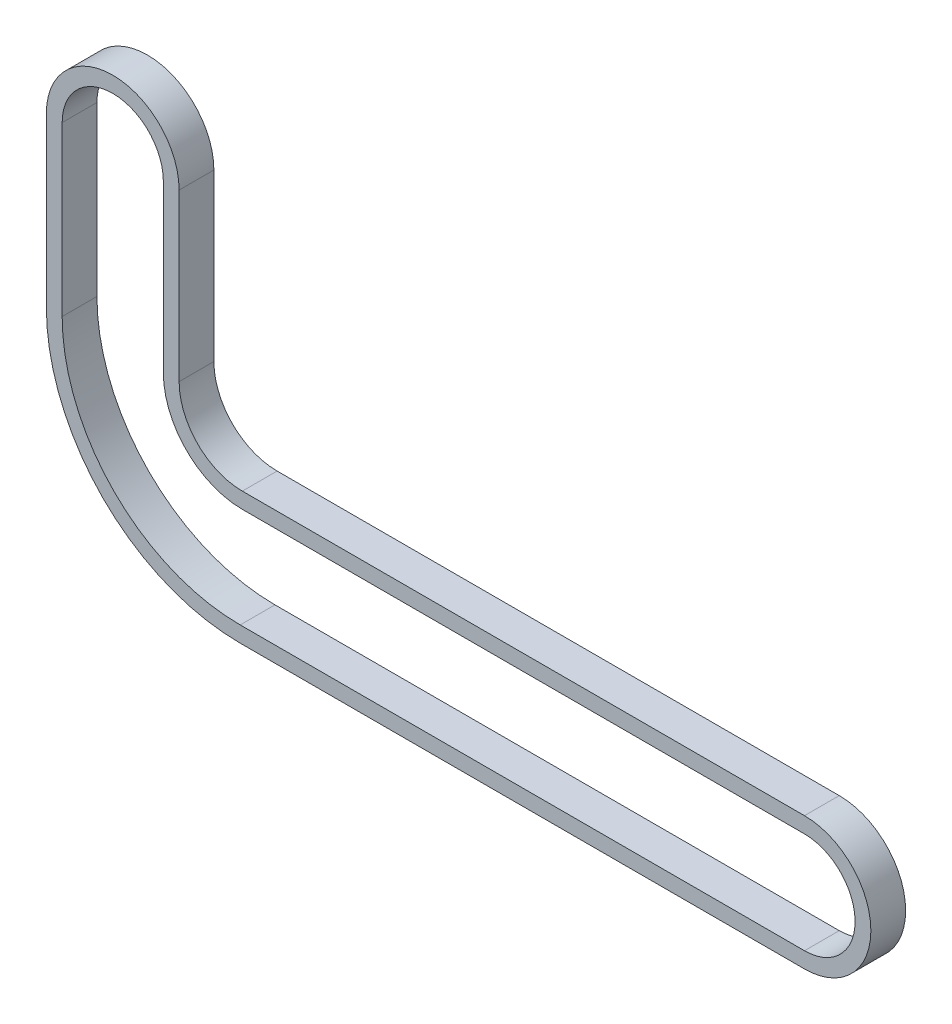
SolidWorks part; units mm, degrees
ref_plane "Front Plane" through (0, 0, 0) normal (0, 0, 1) x (1, 0, 0)
ref_plane "Top Plane" through (0, 0, 0) normal (0, 1, 0) x (1, 0, 0)
ref_plane "Right Plane" through (0, 0, 0) normal (1, 0, 0) x (0, 0, -1)
sketch "Sketch1" plane through (0, 0, 0) normal (0, 0, 1) x (1, 0, 0)
  line L0 (-55.3634, 75.858) -> (-55.3634, 22.7074)
  line L1 (0.9629, -33.6189) -> (179.4809, -33.6189)
  line L3 (179.4809, -1.6189) -> (1.6366, -1.6189)
  line L4 (-23.3634, 23.3811) -> (-23.3634, 75.858)
  line L5 (-18.3634, 23.3811) -> (-18.3634, 75.858)
  line L6 (-60.3634, 75.858) -> (-60.3634, 22.7074)
  line L7 (0.9629, -38.6189) -> (179.4809, -38.6189)
  line L8 (179.4809, 3.3811) -> (1.6366, 3.3811)
  arc A0 (179.4809, -1.6189) -> (179.4809, -33.6189) centre (179.4809, -17.6189) cw
  arc A1 (-55.3634, 22.7074) -> (0.9629, -33.6189) centre (0.9629, 22.7074) ccw
  arc A2 (-55.3634, 75.858) -> (-23.3634, 75.858) centre (-39.3634, 75.858) cw
  arc A3 (1.6366, -1.6189) -> (-23.3634, 23.3811) centre (1.6366, 23.3811) cw
  arc A4 (-60.3634, 75.858) -> (-18.3634, 75.858) centre (-39.3634, 75.858) cw
  arc A5 (-60.3634, 22.7074) -> (0.9629, -38.6189) centre (0.9629, 22.7074) ccw
  arc A6 (179.4809, 3.3811) -> (179.4809, -38.6189) centre (179.4809, -17.6189) cw
  arc A7 (1.6366, 3.3811) -> (-18.3634, 23.3811) centre (1.6366, 23.3811) cw
  arc A8 (1.6366, -1.6189) -> (-23.3634, 23.3811) centre (1.6366, 23.3811) cw construction
  dimension "D1" = 16
  dimension "D2" = 16
  dimension "D3" = 25
  dimension "D4" = 5
extrude "Boss-Extrude1" add sketch "Sketch1" against normal blind 11
